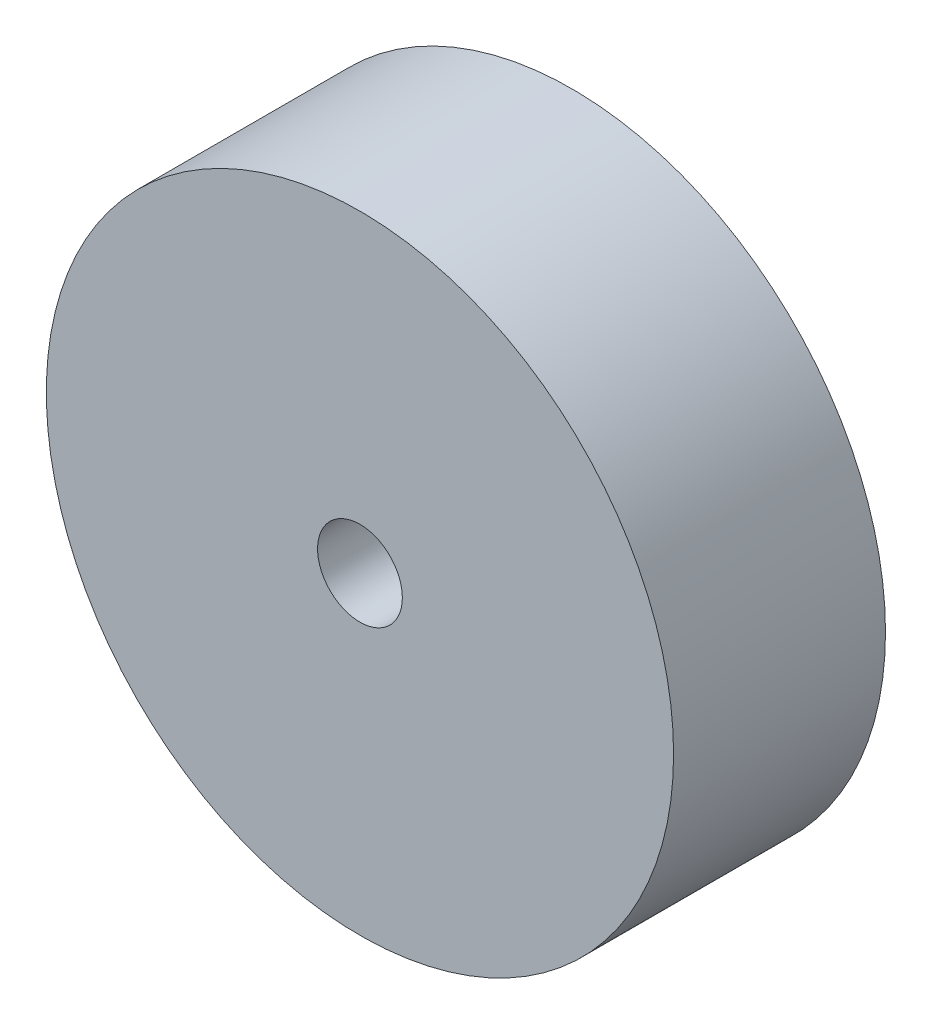
SolidWorks part; units mm, degrees
ref_plane "Front Plane" through (0, 0, 0) normal (0, 0, 1) x (1, 0, 0)
ref_plane "Top Plane" through (0, 0, 0) normal (0, 1, 0) x (1, 0, 0)
ref_plane "Right Plane" through (0, 0, 0) normal (1, 0, 0) x (0, 0, -1)
other "Configuration Table"
sketch "Sketch1" plane through (0, 0, 0) normal (0, 0, 1) x (1, 0, 0)
  circle A0 centre (0, 0) radius 7.4
  circle A1 centre (0, 0) radius 1
  dimension "D1" = 14.8
  dimension "D2" = 2
extrude "Boss-Extrude1" add sketch "Sketch1" along normal blind 5
sketch "Sketch2" plane through (0, 0, 5) normal (0, 0, 1) x (1, 0, 0)
  line L0 (0, 0) -> (7.4, 0) construction
  circle A0 centre (0, 0) radius 7.4 construction
